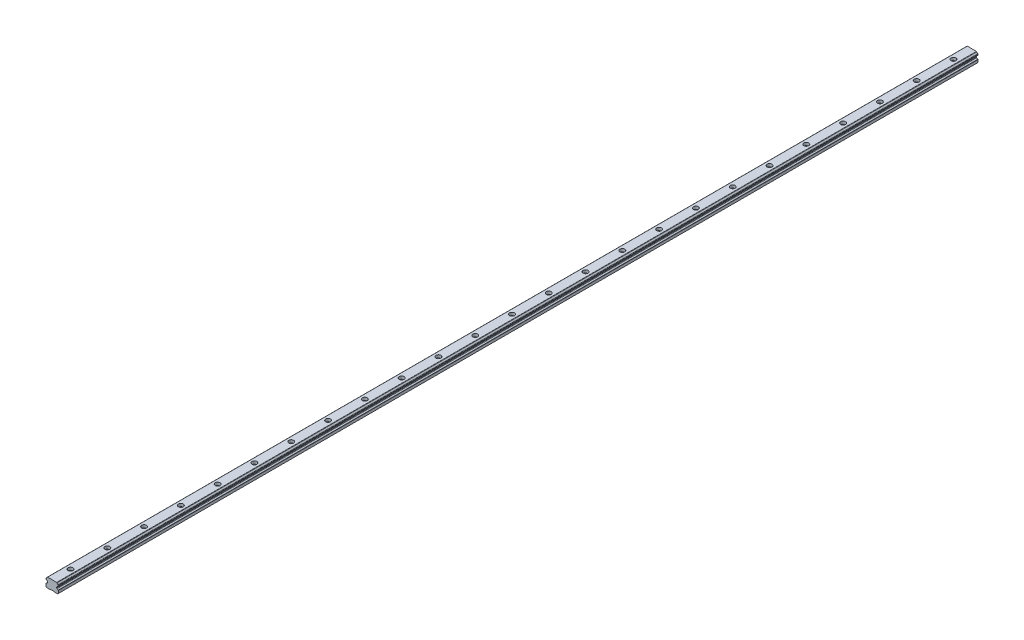
from build123d import *

# Parameters (mm, degrees)
EXTRUDE_1_DEPTH           = 750
HOLE_WIZARD_1_D           = 4.5
HOLE_WIZARD_1_CBORE_D     = 8
HOLE_WIZARD_1_CBORE_DEPTH = 4.6
PATTERN_LINEAR_1_COUNT    = 25
PATTERN_LINEAR_1_PITCH    = 60


with BuildPart() as part:
    # 草图1 → 凸台-拉伸1 (new, symmetric)
    with BuildSketch(Plane.XY):
        with BuildLine():
            Line((-9, -15.5), (-3, -15.5))
            Line((-3, -15.5), (-3, -15))
            Line((-3, -15), (3, -15))
            Line((3, -15), (3, -15.5))
            Line((3, -15.5), (9, -15.5))
            Line((9, -15.5), (10, -14.5))
            Line((10, -14.5), (10, -10.283095189))
            ThreePointArc((10, -10.283095189), (9.935099953, -10.036745782), (9.757247878, -9.854348727))
            Line((9.757247878, -9.854348727), (7.985504245, -8.791302547))
            ThreePointArc((7.985504245, -8.791302547), (7.629800093, -8.426508436), (7.5, -7.933809621))
            Line((7.5, -7.933809621), (7.5, -6.728314441))
            ThreePointArc((7.5, -6.728314441), (7.54517441, -6.52062794), (7.672534731, -6.3504699))
            Line((7.672534731, -6.3504699), (7.722596238, -6.307083261))
            ThreePointArc((7.722596238, -6.307083261), (7.824957798, -6.184677355), (7.883543912, -6.036256459))
            ThreePointArc((7.883543912, -6.036256459), (8.488825425, -4.947326226), (9.59375, -4.371760027))
            ThreePointArc((9.59375, -4.371760027), (9.885275875, -4.199316445), (10, -3.880627726))
            Line((10, -3.880627726), (10, -2.619372274))
            ThreePointArc((10, -2.619372274), (9.885275875, -2.300683555), (9.59375, -2.128239973))
            ThreePointArc((9.59375, -2.128239973), (8.467935307, -1.532064693), (7.871760027, -0.40625))
            ThreePointArc((7.871760027, -0.40625), (7.699316445, -0.114724125), (7.380627726, 0))
            Line((7.380627726, 0), (-7.380627726, 0))
            ThreePointArc((-7.380627726, 0), (-7.699316445, -0.114724125), (-7.871760027, -0.40625))
            ThreePointArc((-7.871760027, -0.40625), (-8.467935307, -1.532064693), (-9.59375, -2.128239973))
            ThreePointArc((-9.59375, -2.128239973), (-9.885275875, -2.300683555), (-10, -2.619372274))
            Line((-10, -2.619372274), (-10, -3.880627726))
            ThreePointArc((-10, -3.880627726), (-9.885275875, -4.199316445), (-9.59375, -4.371760027))
            ThreePointArc((-9.59375, -4.371760027), (-8.488825425, -4.947326226), (-7.883543912, -6.036256459))
            ThreePointArc((-7.883543912, -6.036256459), (-7.824957798, -6.184677355), (-7.722596238, -6.307083261))
            Line((-7.722596238, -6.307083261), (-7.672534731, -6.3504699))
            ThreePointArc((-7.672534731, -6.3504699), (-7.54517441, -6.52062794), (-7.5, -6.728314441))
            Line((-7.5, -6.728314441), (-7.5, -7.933809621))
            ThreePointArc((-7.5, -7.933809621), (-7.629800093, -8.426508436), (-7.985504245, -8.791302547))
            Line((-7.985504245, -8.791302547), (-9.757247878, -9.854348727))
            ThreePointArc((-9.757247878, -9.854348727), (-9.935099953, -10.036745782), (-10, -10.283095189))
            Line((-10, -10.283095189), (-10, -14.5))
            Line((-10, -14.5), (-9, -15.5))
        make_face()
    extrude(amount=EXTRUDE_1_DEPTH, both=True)

    # 打孔尺寸(%根据)内六角圆柱头螺钉的类型1 (through all)
    with Locations(Plane(origin=(0, 0, 720), x_dir=(0, 0, 1), z_dir=(0, 1, 0))):
        with Locations((0, 0)):
            hole_wizard_1 = CounterBoreHole(HOLE_WIZARD_1_D / 2, HOLE_WIZARD_1_CBORE_D / 2, HOLE_WIZARD_1_CBORE_DEPTH)

    # 阵列(线性)1: 打孔尺寸(%根据)内六角圆柱头螺钉的类型1 ×25
    with Locations(*[(0, 0, -i * PATTERN_LINEAR_1_PITCH) for i in range(1, PATTERN_LINEAR_1_COUNT)]):
        add(hole_wizard_1, mode=Mode.SUBTRACT)


solid = part.part
